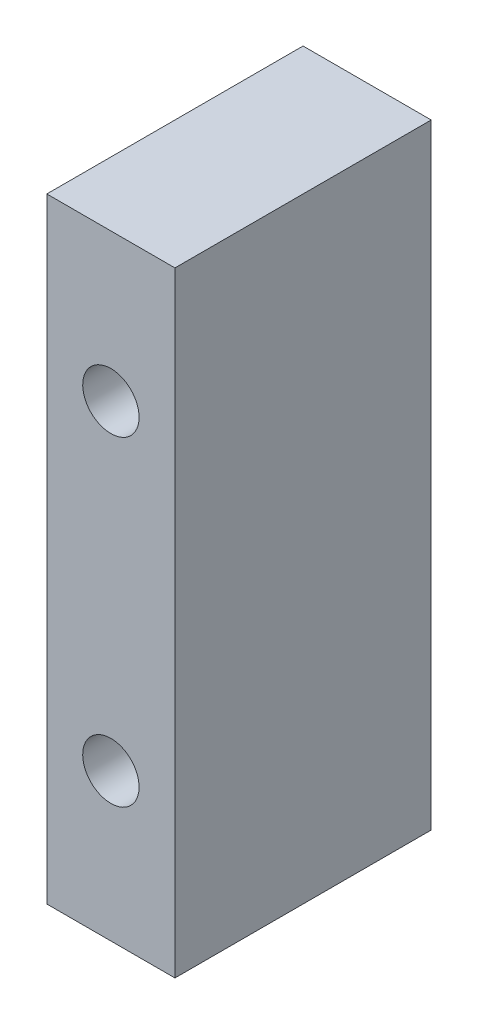
from build123d import *

# Parameters (mm, degrees)
SKETCH_1_W                = 20
SKETCH_1_H                = 48
EXTRUDE_1_DEPTH           = 10
HOLE_WIZARD_1_D           = 4.4
HOLE_WIZARD_1_CBORE_D     = 8
HOLE_WIZARD_1_CBORE_DEPTH = 5


with BuildPart() as part:
    # 草图1 → 凸台-拉伸1 (new body)
    with BuildSketch(Plane(origin=(0, 0, 0), x_dir=(0, 0, -1), z_dir=(1, 0, 0))):
        Rectangle(SKETCH_1_W, SKETCH_1_H)
    extrude(amount=EXTRUDE_1_DEPTH)

    # 打孔尺寸(%根据)内六角圆柱头螺钉的类型1 (through all)
    with Locations(Plane(origin=(0, 0, -10), x_dir=(-1, 0, 0), z_dir=(0, 0, -1))):
        with Locations((-5, -12.5), (-5, 12.5)):
            CounterBoreHole(HOLE_WIZARD_1_D / 2, HOLE_WIZARD_1_CBORE_D / 2, HOLE_WIZARD_1_CBORE_DEPTH)


solid = part.part
